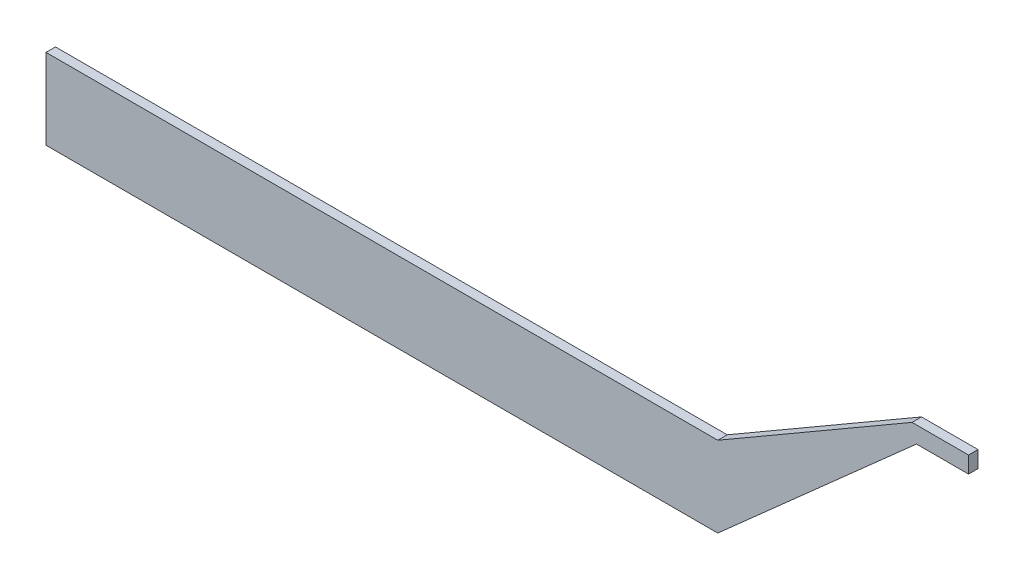
from build123d import *

# Parameters (mm, degrees)
BOSS_EXTRUDE1_DEPTH = 0.2


with BuildPart() as part:
    # Sketch1 → Boss-Extrude1 (new body)
    with BuildSketch(Plane.XY):
        Polygon((14.2, 1.7), (18.305715448, 4.08), (19.5, 4.08), (19.5, 3.73), (18.4, 3.73), (14.19879989, 0), (0, 0), (0, 1.7), align=None)
    extrude(amount=BOSS_EXTRUDE1_DEPTH)


solid = part.part
